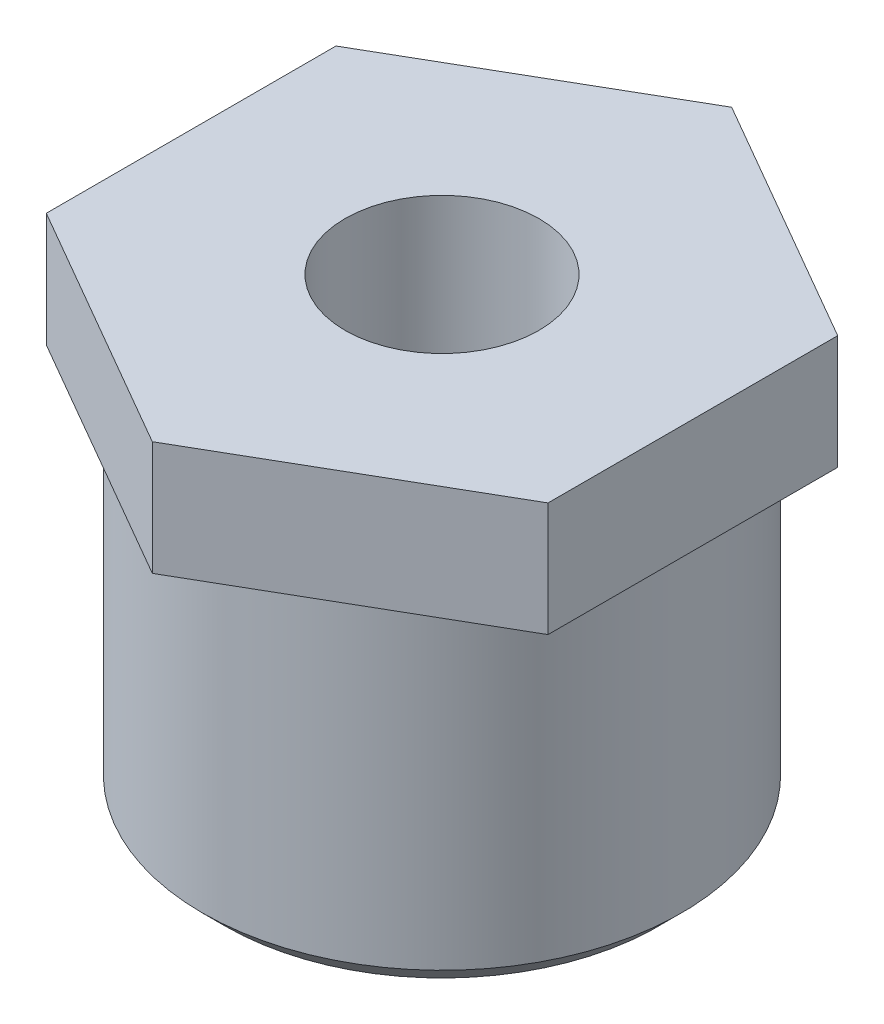
SolidWorks part; units mm, degrees
material "AISI 304"
ref_plane "Front Plane" through (0, 0, 0) normal (0, 0, 1) x (1, 0, 0)
ref_plane "Top Plane" through (0, 0, 0) normal (0, 1, 0) x (1, 0, 0)
ref_plane "Right Plane" through (0, 0, 0) normal (1, 0, 0) x (0, 0, -1)
sketch "Sketch1" plane through (0, 0, 0) normal (0, 1, 0) x (1, 0, 0)
  line L1 (11, -6.3509) -> (11, 6.3509)
  line L2 (11, 6.3509) -> (0, 12.7017)
  line L3 (0, 12.7017) -> (-11, 6.3509)
  line L4 (-11, 6.3509) -> (-11, -6.3509)
  line L5 (-11, -6.3509) -> (0, -12.7017)
  line L6 (0, -12.7017) -> (11, -6.3509)
  circle A0 centre (0, 0) radius 11 construction
  dimension "D1" = 22
extrude "Boss-Extrude1" add sketch "Sketch1" along normal blind 20
sketch "Sketch3" plane through (0, 0, 0) normal (0, -1, 0) x (1, 0, 0)
  circle A0 centre (0, 0) radius 10.5
  dimension "D1" = 21
extrude "Cut-Extrude1" cut sketch "Sketch3" against normal offset from surface (15 mm away) 5 flip side to cut up to face at (0, 20, 0)
cosmetic thread "Cosmetic Thread1" parameters "D2"=18.631
chamfer "Chamfer1" distance 1 angle 45 1 edges at (0, 0, -10.5)
sketch "Sketch9" plane through (0, 20, 0) normal (0, 1, 0) x (1, 0, 0)
  point P0 (0, 0)
hole_wizard "M10 Tapped Hole1" positions "3DSketch1" profile "Sketch10" tap size "M10" standard "GB" end condition through all
sketch3d "3DSketch1"
  point P0 (0, 20, 0)
sketch "Sketch10" plane through (0, 20, 0) normal (1, 0, 0) x (0, 0, 1)
  line L0 (0, 0) -> (0, 20)
  line L1 (0, 20) -> (4.25, 20)
  line L2 (4.25, 20) -> (4.25, 0)
  line L5 (4.25, 0) -> (0, 0)
  line L11 (0, -6.35) -> (0, 107.95) construction
  dimension "通孔螺纹孔钻头直径" = 8.5
  dimension "通孔螺纹孔钻头深度" = 20
cosmetic thread "Hole Cosmetic Thread1" parameters "D2"=10
